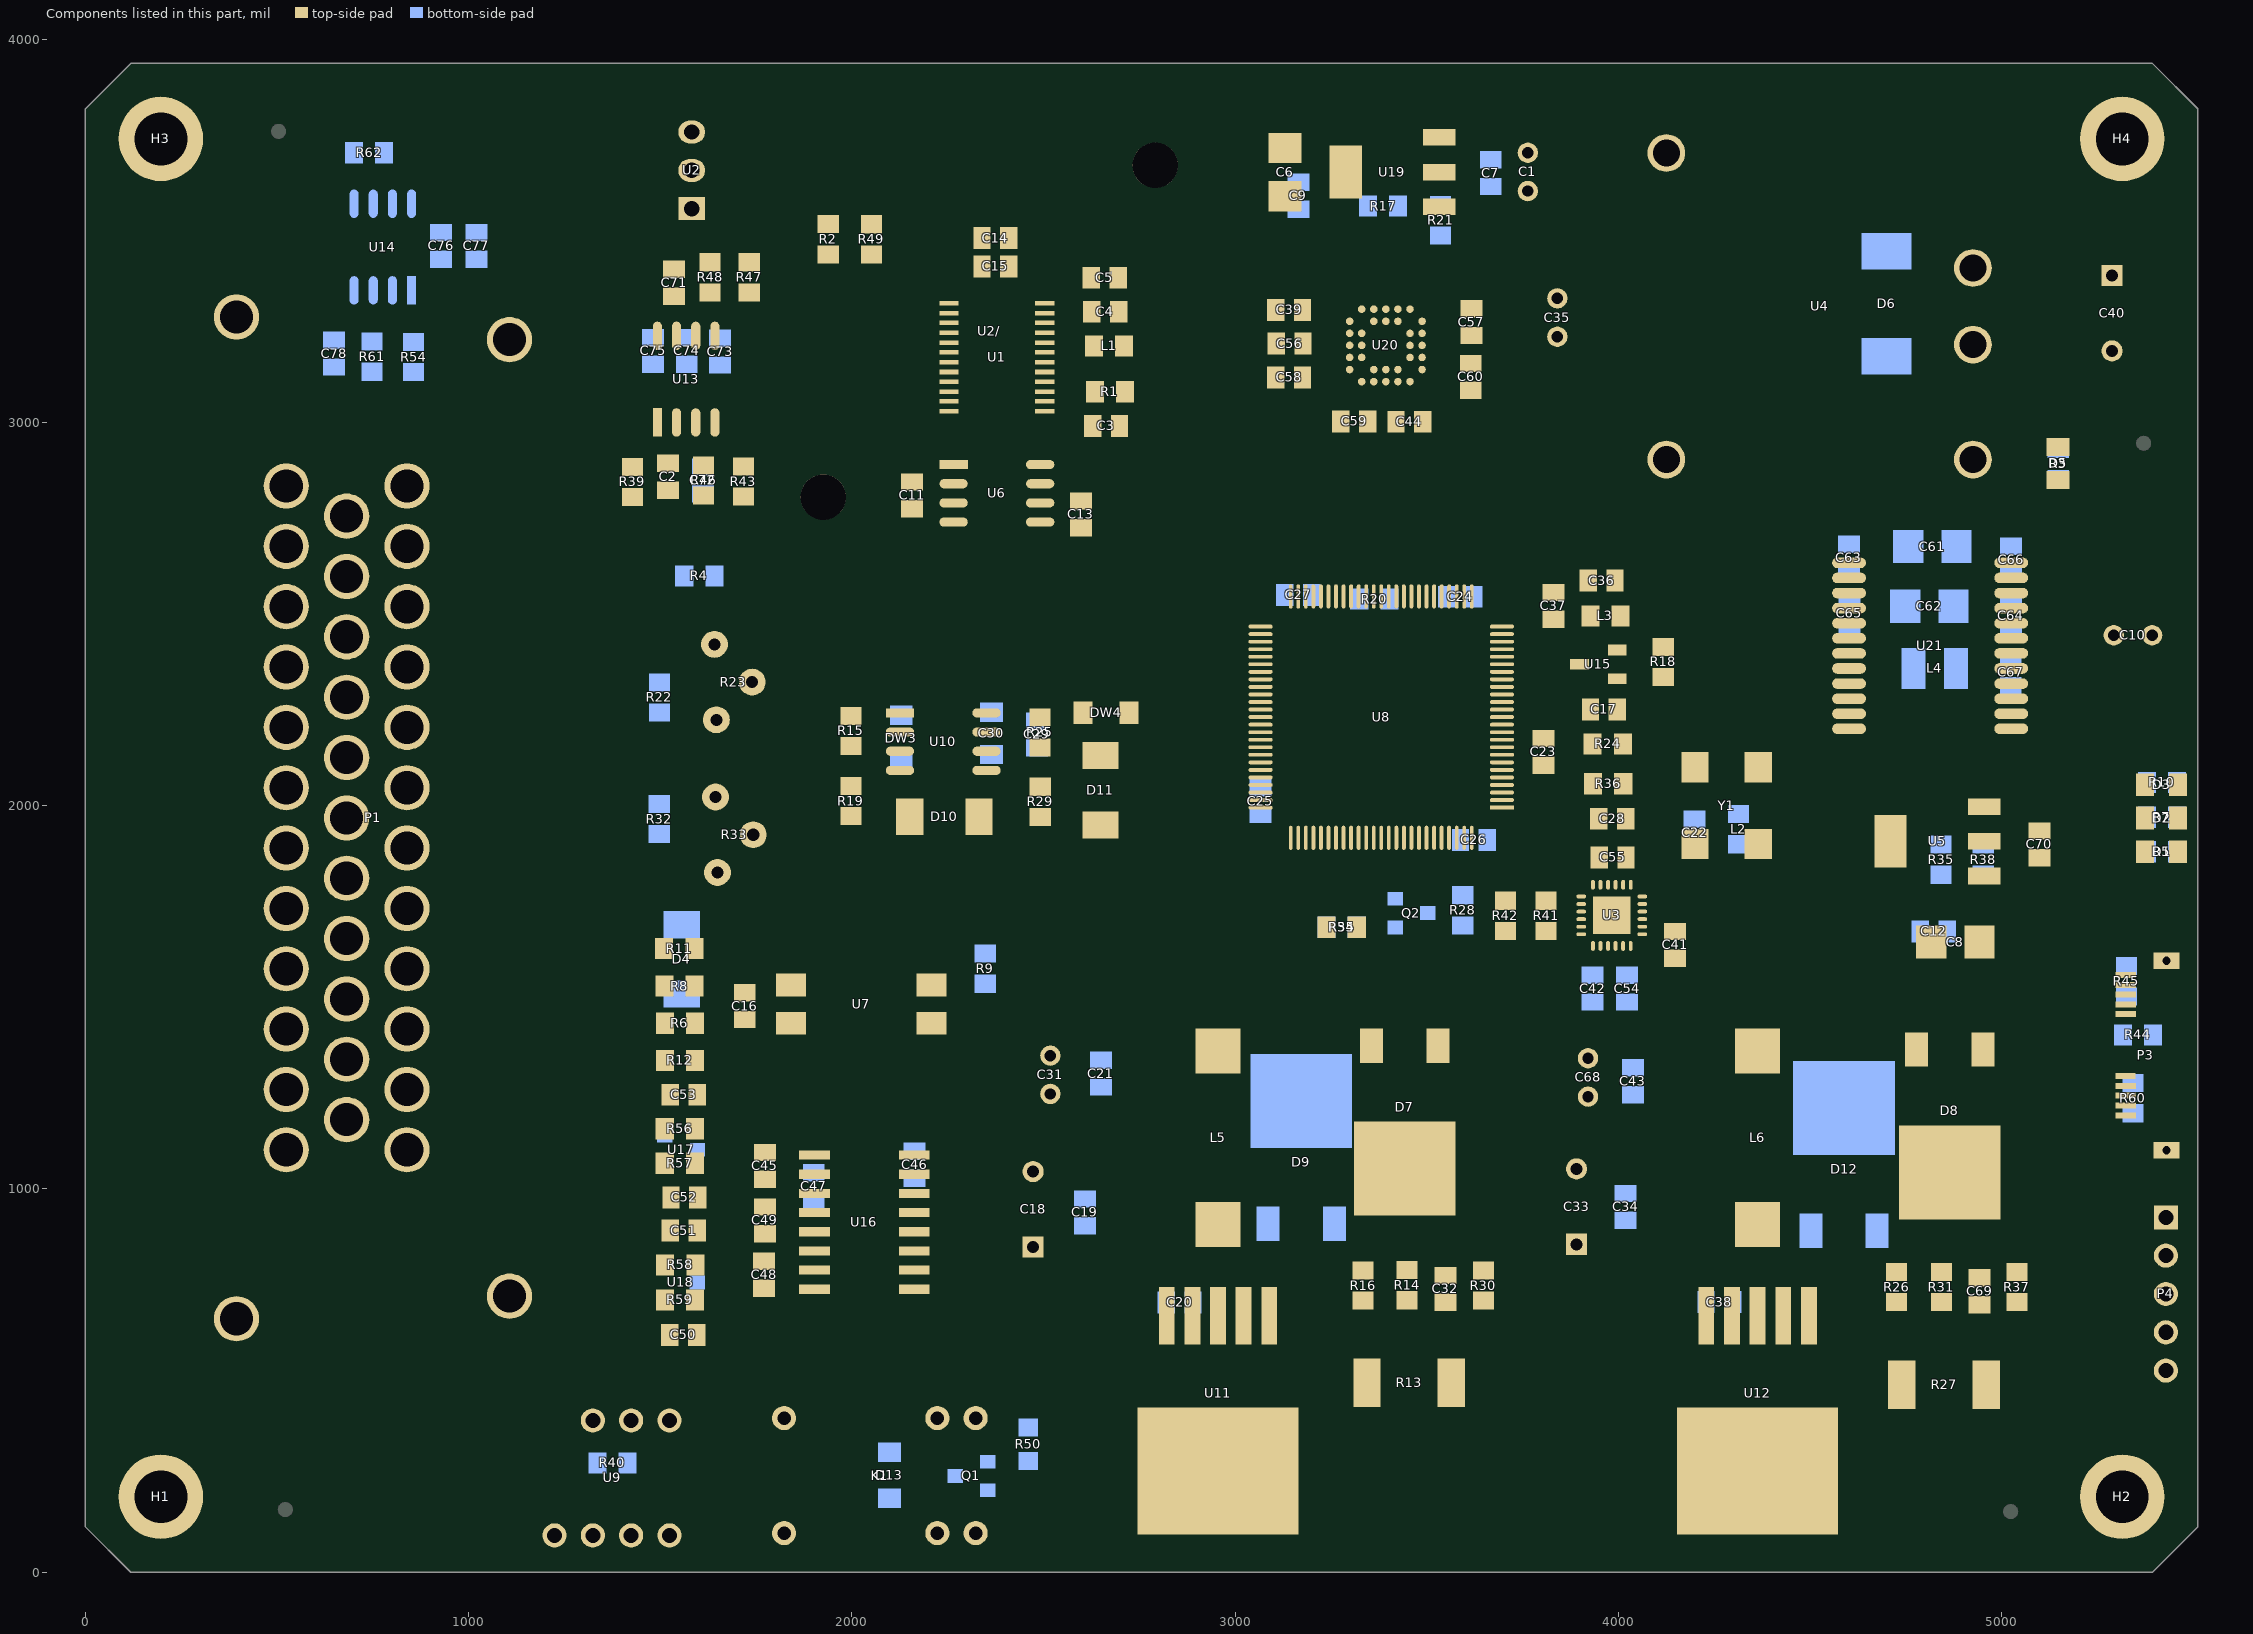
[diagram p0: the components of this part, seen from the top]
# Altium PCB MISC82155.PcbDoc (part 5 of 5)
Units mil, origin at the board's own origin, x right, y up, seen from the top; angles counter-clockwise.
Board outline 5511.81 x 3937.01 mil, 4 copper layers (Top Layer, GND, POWER, Bottom Layer); 191 components, 134 nets, 709 pads, 440 vias.

## Polygon pours and split planes (outlines as drawn) (continued)
GND_SB on Top Layer "Top Layer-No Net" (solid, remove dead copper, pour order 16): 4680,701 4680,423 4688,415 4691,412 4722,412 4774,412 4781,419 4786,424 4786,442 4786,646 4769,663 4760,672 4760,692 4760,727 4757,730 4746,730 4688,730 4680,722 4680,701
NetD7_2 on Top Layer "Top Layer-No Net" (solid, remove dead copper, pour order 14): 2926,745 2926,596 2930,592 2932,590 2940,590 2981,590 2985,594 2986,595 2986,607 2986,787 3022,823 3097,898 3423,898 3563,898 3580,915 3590,925 3590,985 3590,1172 3582,1180 3580,1182 3546,1182 3259,1182 3221,1144 3132,1055 3063,1055 2952,1055 2918,1021 2881,984 2881,942 2881,821 2907,795 2926,776 2926,745
NetD8_2 on Top Layer "Top Layer-No Net" (solid, remove dead copper, pour order 12): 4284,913 4284,836 4316,804 4339,781 4339,739 4339,594 4343,590 4345,588 4354,588 4383,588 4386,591 4389,594 4389,603 4389,776 4433,820 4496,883 4850,883 4987,883 5004,900 5013,909 5013,972 5013,1165 5004,1174 4998,1180 4983,1180 4711,1180 4679,1148 4519,988 4382,988 4306,988 4288,970 4284,966 4284,913
SO_12V on Top Layer "Top Layer-No Net" (solid, remove dead copper, pour order 10): 2442,915 2442,823 2462,803 2493,772 2493,729 2493,692 2513,672 2601,584 2811,584 2835,584 2842,591 2844,593 2844,600 2844,775 2822,797 2758,861 2712,861 2666,861 2635,892 2584,943 2525,943 2470,943 2442,915
SO_12V on Top Layer "Top Layer-No Net" (solid, remove dead copper, pour order 8): 3855,908 3854,907 3854,830 3854,809 3909,754 4086,577 4200,577 4242,577 4252,587 4253,588 4253,620 4253,778 4240,791 4231,800 4206,800 4092,800 3998,894 3960,932 3918,932 3879,932 3855,908
VDD_12V on Top Layer "Top Layer-No Net" (solid, remove dead copper, pour order 4): 3483,3782 3483,3739 3483,3726 3487,3722 3488,3721 3499,3721 3681,3721 3705,3697 3729,3673 3777,3673 3797,3673 3876,3752 3928,3804 4520,3804 4612,3804 4679,3737 4803,3613 4803,3468 4803,3402 4850,3355 4859,3346 5003,3346 5324,3346 5341,3363 5345,3367 5345,3393 5345,3455 5326,3474 5286,3514 5245,3514 5187,3514 5103,3598 4791,3910 4244,3910 3739,3910 3716,3887 3681,3852 3610,3852 3513,3852 3494,3833 3483,3822 3483,3782
VDD_3.3 on Top Layer "Top Layer-No Net" (solid, remove dead copper, pour order 2): 3291,1711 3291,1664 3291,1656 3295,1652 3296,1651 3310,1651 3349,1651 3353,1655 3357,1659 3357,1680 3357,1741 3341,1757 3326,1772 3307,1772 3280,1772 3276,1768 3271,1763 3271,1753 3271,1735 3287,1719 3291,1715 3291,1711
GND on Top Layer "Top Layer-No Net" (solid, remove dead copper, pour order 0): -328.05,4094.29 -328.05,-7.71 -162.05,-173.71 -98.05,-237.71 1410.95,-237.71 5441.95,-237.71 5694.95,15.29 5860.95,181.29 5860.95,1478.29 5860.95,3817.29 5528.95,4149.29 5338.95,4339.29 2651.95,4339.29 -83.05,4339.29 -328.05,4094.29
GND_SB on Bottom Layer "Top Layer-No Net" (solid, remove dead copper, pour order 44): 4630,861 4651,840 4674,817 4674,718 4674,568 4680,562 4685,557 4719,557 4770,557 4783,570 4788,575 4788,615 4788,857 4714,931 4702,943 4680,943 4648,943 4636,931 4630,925 4630,861
GND_SA on Bottom Layer "Top Layer-No Net" (solid, remove dead copper, pour order 42): 3200,886 3228,858 3276,810 3276,713 3276,585 3286,575 3291,570 3322,570 3393,570 3398,575 3401,578 3401,596 3401,861 3315,947 3302,960 3271,960 3213,960 3204,951 3200,947 3200,886
SOLENIOD_A on Bottom Layer "Top Layer-No Net" (solid, remove dead copper, pour order 40): 2465,1388 2465,1331 2478,1318 2490,1306 2575,1306 2826,1306 2955,1177 3037,1095 3100,1095 3303,1095 3314,1106 3323,1115 3323,1146 3323,1380 3293,1410 3223,1480 3052,1480 2537,1480 2478,1421 2465,1408 2465,1388
SOLENIOD_B on Bottom Layer "Top Layer-No Net" (solid, remove dead copper, pour order 38): 3801,1371 3801,1324 3819,1306 3836,1289 4047,1289 4237,1289 4368,1158 4446,1080 4539,1080 4721,1080 4732,1091 4739,1098 4739,1122 4739,1318 4717,1340 4644,1413 3888,1413 3828,1413 3808,1393 3801,1386 3801,1371
VDD_3.3 on Bottom Layer "Top Layer-No Net" (solid, remove dead copper, pour order 36): 4687,1712 4687,1645 4695,1637 4708,1624 4730,1624 4797,1624 4812.84,1639.85 4816,1643 4816,1664 4816,1702 4814,1704 4814,1712 4807,1719 4804,1722 4756,1722 4697,1722 4687,1712
GND on Bottom Layer "Top Layer-No Net" (solid, remove dead copper, pour order 34): -274.13,4033.8 -274.13,-68.2 -108.13,-234.2 -44.13,-298.2 1464.87,-298.2 5495.87,-298.2 5748.87,-45.2 5914.87,120.8 5914.87,1417.8 5914.87,3756.8 5582.87,4088.8 5392.87,4278.8 2705.87,4278.8 -29.13,4278.8 -274.13,4033.8
GND on GND (split plane): 5491.72,3810.58 5491.72,126.43 5385.38,20.1 126.43,20.1 20.1,126.43 20.1,3810.58 126.43,3916.91 5385.38,3916.91
AGND on GND (split plane): 2186.91,3688.82 2186.91,3287 2187.26,3284.39 2188.27,3281.96 2189.87,3279.87 2321.87,3147.87 2323.96,3146.26 2324.67,3145.97 2326.39,3145.26 2329,3144.91 2421,3144.91 2423.61,3145.26 2426.04,3146.26 2428.13,3147.87 2826.18,3545.91 3381.82,3545.91 3548.91,3378.82 3548.91,3291.18 3526.82,3269.09 3468.18,3269.09 3378.13,3359.13 3376.04,3360.74 3373.61,3361.74 3371,3362.09 3170,3362.09 3167.39,3361.74 3166.68,3361.45 3164.96,3360.74 3162.87,3359.13 2975.87,3172.13 2974.27,3170.04 2973.26,3167.61 2972.91,3165 2972.91,2597.18 2886.87,2511.13 2885.27,2509.04 2884.26,2506.61 2883.91,2504 2883.91,2079.18 2666.82,1862.09 2209,1862.09 2206.39,1861.74 2203.96,1860.74 2201.87,1859.13 1650.82,1308.09 1398.18,1308.09 1197.09,1509.18 1197.09,3440 1197.09,3473.82 1460.18,3736.91 2138.82,3736.91
VDD_12V on POWER (split plane): 5491.72,3810.58 5491.72,3335.09 4953.18,3335.09 4525.13,3763.13 4523.04,3764.74 4520.61,3765.74 4518,3766.09 4020,3766.09 4017.39,3765.74 4015.67,3765.03 4014.96,3764.74 4012.87,3763.13 3856.82,3607.09 3669.18,3607.09 3559.13,3717.13 3557.04,3718.74 3554.61,3719.74 3552,3720.09 1669,3720.09 1666.39,3719.74 1665.17,3719.24 1663.96,3718.74 1661.87,3717.13 1389.87,3445.13 1388.27,3443.04 1387.26,3440.61 1386.91,3438 1386.91,3096.74 1386.77,3096.54 1385.76,3094.11 1385.41,3091.5 1385.76,3088.89 1386.77,3086.46 1388.37,3084.37 1709.87,2762.87 1711.96,2761.26 1714.39,2760.26 1717,2759.91 2136.82,2759.91 2467.91,2428.82 2467.91,2090.18 2207.87,1830.13 2206.27,1828.04 2205.26,1825.61 2204.91,1823 2204.91,1483.09 1317,1483.09 1314.39,1482.74 1311.96,1481.74 1309.87,1480.13 1076.82,1247.09 653.09,1247.09 653.09,1473 652.74,1475.61 651.74,1478.04 650.13,1480.13 601.13,1529.13 599.04,1530.74 596.61,1531.74 594,1532.09 337,1532.09 334.39,1531.74 332.67,1531.03 331.96,1530.74 329.87,1529.13 243.87,1443.13 242.27,1441.04 241.26,1438.61 240.91,1436 240.91,768 241.26,765.39 242.27,762.96 243.87,760.87 625.87,378.87 627.96,377.26 628.67,376.97 630.39,376.26 633,375.91 1569,375.91 1571.61,376.26 1574.04,377.26 1576.13,378.87 1657.13,459.87 1833.38,636.12 1975.91,493.59 1975.91,20.1 126.43,20.1 20.1,126.43 20.1,3810.58 126.43,3916.91 5385.38,3916.91
VDD_5V on POWER (split plane): 4941.87,3317.87 4943.96,3316.26 4946.39,3315.26 4949,3314.91 5491.72,3314.91 5491.72,126.43 5385.38,20.1 4658.09,20.1 4658.09,893 4657.74,895.61 4656.74,898.04 4655.13,900.13 4375.76,1179.5 4805.13,1608.87 4806.74,1610.96 4807.03,1611.67 4807.74,1613.39 4808.09,1616 4808.09,1866.82 5059.13,2117.87 5154.13,2212.87 5155.74,2214.96 5156.24,2216.17 5156.74,2217.39 5157.09,2220 5157.09,2348.5 5157.09,2687 5156.74,2689.61 5156.03,2691.33 5155.74,2692.04 5154.13,2694.13 5068.13,2780.13 5066.04,2781.74 5063.61,2782.74 5061,2783.09 4306,2783.09 4303.39,2782.74 4300.96,2781.74 4298.87,2780.13 4221.87,2703.13 4220.27,2701.04 4219.26,2698.61 4218.91,2696 4218.91,2454.18 4194.82,2430.09 4105.18,2430.09 4091.09,2444.18 4091.09,2473.82 4098.13,2480.87 4099.74,2482.96 4100.45,2484.68 4100.74,2485.39 4101.09,2488 4101.09,2623 4100.74,2625.61 4100.24,2626.83 4099.74,2628.04 4098.13,2630.13 4062.13,2666.13 4060.04,2667.74 4057.61,2668.74 4055,2669.09 2771.18,2669.09 2749.13,2691.13 2696.59,2743.68 2696.59,3041.5 2696.24,3044.11 2695.24,3046.54 2693.63,3048.63 2612.09,3130.18 2612.09,3328 2611.74,3330.61 2610.74,3333.04 2609.13,3335.13 2528.13,3416.13 2526.04,3417.74 2523.61,3418.74 2521,3419.09 2275,3419.09 2272.39,3418.74 2269.96,3417.74 2267.87,3416.13 2173.87,3322.13 2172.27,3320.04 2171.26,3317.61 2170.91,3315 2170.91,2814.18 2136.82,2780.09 1721.18,2780.09 1407.09,3094.18 1407.09,3433.82 1673.18,3699.91 3547.82,3699.91 3657.87,3589.87 3659.96,3588.26 3661.68,3587.55 3662.39,3587.26 3665,3586.91 3861,3586.91 3863.61,3587.26 3866.04,3588.26 3868.13,3589.87 4024.18,3745.91 4513.82,3745.91
VDD_3.3 on POWER (split plane): 2591.91,3323.82 2591.91,3126 2592.26,3123.39 2593.27,3120.96 2594.87,3118.87 2676.41,3037.32 2676.41,2739.5 2676.76,2736.89 2677.77,2734.46 2679.37,2732.37 2734.87,2676.87 2759.87,2651.87 2761.96,2650.26 2763.68,2649.55 2764.39,2649.26 2767,2648.91 4050.82,2648.91 4080.91,2618.82 4080.91,2492.18 4073.87,2485.13 4072.27,2483.04 4071.26,2480.61 4070.91,2478 4070.91,2440 4071.26,2437.39 4072.27,2434.96 4073.87,2432.87 4093.87,2412.87 4095.96,2411.26 4098.39,2410.26 4101,2409.91 4199,2409.91 4201.61,2410.26 4204.04,2411.26 4206.13,2412.87 4236.13,2442.87 4237.74,2444.96 4238.74,2447.39 4239.09,2450 4239.09,2691.82 4310.18,2762.91 5056.82,2762.91 5136.91,2682.82 5136.91,2348.5 5136.91,2224.18 5044.87,2132.13 4790.87,1878.13 4789.27,1876.04 4788.26,1873.61 4787.91,1871 4787.91,1620.18 4353.82,1186.09 3968.18,1186.09 3930.13,1224.13 3929.09,1224.93 3929.09,1380 3928.74,1382.61 3928.03,1384.33 3927.74,1385.04 3926.13,1387.13 3884.13,1429.13 3882.04,1430.74 3879.61,1431.74 3877,1432.09 2703.18,1432.09 2675.13,1460.13 2655.13,1480.13 2653.04,1481.74 2650.61,1482.74 2648,1483.09 2225.09,1483.09 2225.09,1818.82 2485.13,2078.87 2486.74,2080.96 2487.03,2081.67 2487.74,2083.39 2488.09,2086 2488.09,2433 2487.74,2435.61 2487.03,2437.33 2486.74,2438.04 2485.13,2440.13 2155.26,2770 2188.13,2802.87 2189.74,2804.96 2190.45,2806.68 2190.74,2807.39 2191.09,2810 2191.09,3310.82 2279.18,3398.91 2516.82,3398.91
SO_12V on POWER (split plane): 3956.87,1168.87 3958.96,1167.26 3959.67,1166.97 3961.39,1166.26 3964,1165.91 4360.82,1165.91 4637.91,888.82 4637.91,20.1 1996.09,20.1 1996.09,497.76 1995.74,500.37 1995.33,501.38 1994.74,502.81 1993.13,504.9 1847.65,650.38 2144.18,946.91 3659,946.91 3661.61,947.26 3664.04,948.26 3666.13,949.87 3921,1204.74
SOLENIOD_B on POWER (split plane): 632.91,1468.82 632.91,1247.09 478,1247.09 475.39,1246.74 472.96,1245.74 470.87,1244.13 394.87,1168.13 393.27,1166.04 392.26,1163.61 391.91,1161 391.91,1043 392.26,1040.39 393.27,1037.96 394.87,1035.87 565.91,864.82 565.91,807 566.26,804.39 567.27,801.96 568.87,799.87 687.87,680.87 689.96,679.26 692.39,678.26 695,677.91 962,677.91 964.61,678.26 967.04,679.26 969.13,680.87 1451.18,1162.91 2551,1162.91 2553.61,1163.26 2556.04,1164.26 2558.13,1165.87 2675.13,1282.87 2676.74,1284.96 2677.03,1285.67 2677.74,1287.39 2678.09,1290 2678.09,1360 2678.09,1383.82 2706.13,1411.87 2706.17,1411.91 3872.82,1411.91 3908.91,1375.82 3908.91,1221.18 3654.82,967.09 2140,967.09 2137.39,966.74 2134.96,965.74 2132.87,964.13 1642.87,474.13 1564.82,396.09 637.18,396.09 261.09,772.18 261.09,1431.82 341.18,1511.91 589.82,1511.91
SOLENIOD_A on POWER (split plane): 2660.87,1445.87 2686.24,1420.5 2660.87,1395.13 2659.27,1393.04 2658.26,1390.61 2657.91,1388 2657.91,1360 2657.91,1294.18 2546.82,1183.09 1447,1183.09 1444.39,1182.74 1442.67,1182.03 1441.96,1181.74 1439.87,1180.13 957.82,698.09 699.18,698.09 586.09,811.18 586.09,869 585.74,871.61 585.03,873.33 584.74,874.04 583.13,876.13 412.09,1047.18 412.09,1156.82 482.18,1226.91 1081,1226.91 1083.61,1227.26 1086.04,1228.26 1088.13,1229.87 1321.18,1462.91 2643.82,1462.91
VDD_6V on POWER (split plane): 3411.91,3324.82 3411.91,3194 3412.26,3191.39 3413.27,3188.96 3414.87,3186.87 3574.91,3026.82 3574.91,2921.18 3510.82,2857.09 3315.18,2857.09 3090.09,3082.18 3090.09,3515.82 3119.18,3544.91 3191.82,3544.91

## Keep-outs
Keep-Out Layer:
  circle w5: c5023.94,158 r59.06
  circle w5: c503.94,3760 r59.06
  circle w5: c5370.94,2946 r59.06
  circle w5: c521.47,163.34 r59.06
  lines w5: 0,118.11 118.11,0 5393.7,0 5511.81,118.11 5511.81,3818.9 5393.7,3937.01 118.11,3937.01 0,3818.9 0,118.11

## Other copper
Top Layer:
  pour cut-out: 3255.41,3339.34 3255.41,3063.34 3259.41,3059.34 3260.41,3060.34 3534.41,3060.34 3534.41,3341.34 3532.41,3339.34
GND (plane layer: these items are gaps in the copper):
  lines w20: 1187,1505 1187,3440 1187,3478 1456,3747 2143,3747 2197,3693 2197,3287 2329,3155 2421,3155 2822,3556 3386,3556 3559,3383 3559,3287 3531,3259 3464,3259 3371,3352 3170,3352 2983,3165 2983,2593 2894,2504 2894,2075 2671,1852 2209,1852 1655,1298 1394,1298 1187,1505
POWER (plane layer: these items are gaps in the copper):
  lines w20: 407,1522 337,1522 ; 643,1237 643,1473 594,1522 337,1522 ; 1395.5,3091.5 1717,2770 2141,2770 ; 1397,3093 1397,3438 1669,3710 3552,3710 3665,3597 3861,3597 4020,3756 4518,3756 4949,3325 5511.81,3325 ; 1833.38,650.38 1986,497.76 1986,0 ; 2215,1473 2215,1823 2478,2086 2478,2433 2141,2770 ; 2668,1360 2668,1290 ; 3923,1217 3964,1176 4358,1176 ; 4648,18 4648,893 4365,1176 4358,1176 ; 337,1522 251,1436 251,768 633,386 1569,386 1650,467 2140,957 3659,957 3919,1217 3919,1380 3877,1422 2699,1422 ; 2141,2770 2181,2810 2181,3315 2275,3409 2521,3409 2602,3328 2602,3126 2686.5,3041.5 2686.5,2739.5 2742,2684 2767,2659 4055,2659 4091,2623 4091,2488 4081,2478 4081,2440 4101,2420 4199,2420 4229,2450 4229,2696 4306,2773 5061,2773 5147,2687 5147,2348.5 5147,2220 5052,2125 4798,1871 4798,1616 4358,1176 ; 2668,1290 2551,1173 1447,1173 962,688 695,688 576,807 576,869 402,1043 402,1161 478,1237 1081,1237 1317,1473 2357,1473 2648,1473 2668,1453 2699,1422 ; 2668,1290 2668,1388 2699,1419 2699,1422 ; 3080,3078 3080,3520 3115,3555 3196,3555 3422,3329 3422,3194 3585,3031 3585,2917 3515,2847 3311,2847 3080,3078

## Silkscreen, mask and mechanical layers (free items; w line width, h text height)
Top Overlay:
  text "TXD1" at 5232,918 h40
  text "RXD1" at 5248,812 h40
  text "GND" at 5254,714 h40
  text "GND" at 5256,613 h40
  text "BOOT0" at 5199,506 h40
  text "Ctrl_Board" at 583,318 h40
  text "Ver:0.5A" at 895,313 h40
  text "2018-03-05" at 633,173 h40
Bottom Overlay:
  text "GND" at 329,2825 h40
  text "SEAT_SEN" at 1195,2815 h40
  text "GND" at 609,2739 h40
  text "GND" at 330,2665 h40
  text "VDD_12V" at 1163,2661 h40
  text "GND" at 613,2584 h40
  text "FOOT_SW" at 1161,2502 h40
  text "GND" at 331,2501 h40
  text "GND" at 614,2428 h40
  text "GND" at 333,2344 h40
  text "STWHEEL_SEN" at 1291,2343 h40
  text "GND" at 612,2269 h40
  text "VDD_12V" at 1173,2187 h40
  text "GND" at 333,2185 h40
  text "GND" at 608,2112 h40
  text "GND" at 1040,2038 h40
  text "GND" at 336,2031 h40
  text "GND" at 610,1956 h40
  text "VDD_12V" at 414,1875 h40
  text "GND" at 1037,1870 h40
  text "GND" at 610,1795 h40
  text "BOOT0" at 1102,1730 h40
  text "VDD_12V" at 415,1719 h40
  text "CANL" at 614,1640 h40
  text "GND_SB" at 406,1564 h40
  text "COM2_RXD" at 1226,1557 h40
  text "CANL" at 610,1482 h40
  text "COM2_TXD" at 1221,1403 h40
  text "SOLENIOD_B" at 446,1401 h40
  text "CANH" at 614,1324 h40
  text "COM1_RXD" at 1229,1251 h40
  text "GND_SA" at 402,1247 h40
  text "CANH" at 614,1166 h40
  text "COM1_TXD" at 1213,1117 h40
  text "SOLENIOD_A" at 456,1084 h40
Mechanical 2:
  circle w5: c393.3,3275.25 r39.37
  circle w5: c1105.89,3216.2 r39.37
  circle w5: c393.3,661.08 r39.37
  circle w5: c1105.89,720.13 r39.37
  circle w5: c393.7,3275.59 r39.37
  circle w5: c1106.3,3216.54 r39.37
  circle w5: c393.7,661.42 r39.37
  circle w5: c1106.3,720.47 r39.37
  lines w5: -0.41,117.77 -0.41,3818.56 117.7,3936.67 5393.3,3936.67 5511.41,3818.56 5511.41,117.77 5393.3,-0.34 117.7,-0.34 -0.41,117.77
  text "鐏?" at 21813.49,630.78 h40
Mechanical 3:
  lines w5: 5452.35,1928.79 5452.35,2007.53 5491.72,2007.53 5491.72,1928.79 5452.35,1928.79
Mechanical 4:
  lines w5: -0.41,1968.16 5511.41,1968.16